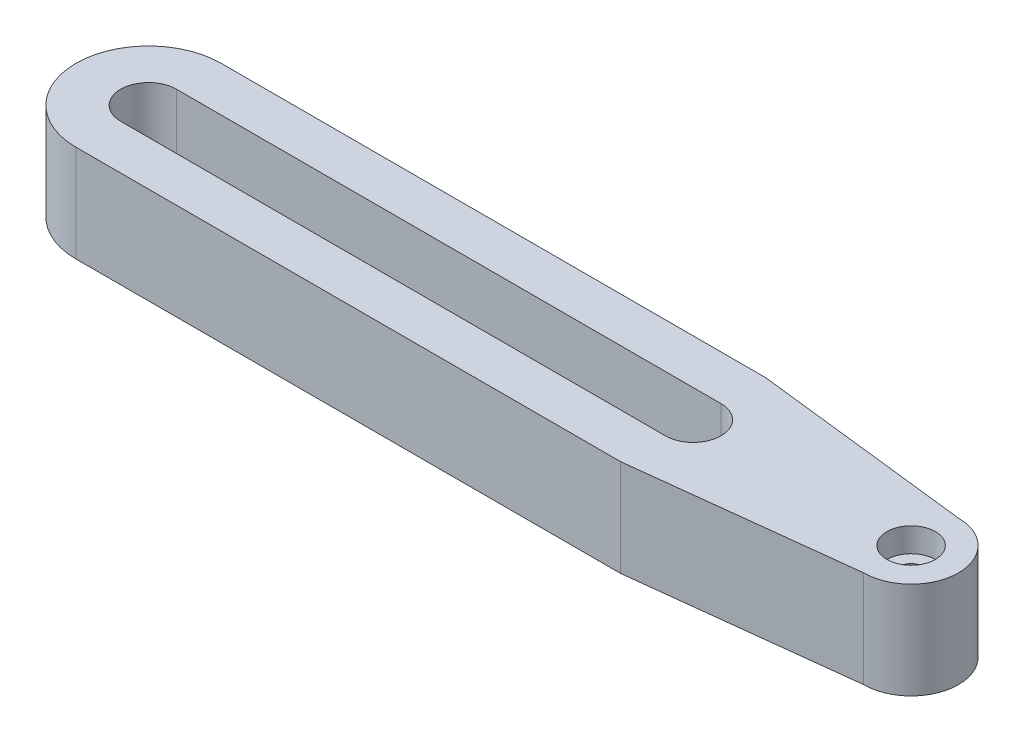
SolidWorks part; units mm, degrees
ref_plane "Front Plane" through (0, 0, 0) normal (0, 0, 1) x (1, 0, 0)
ref_plane "Top Plane" through (0, 0, 0) normal (0, 1, 0) x (1, 0, 0)
ref_plane "Right Plane" through (0, 0, 0) normal (1, 0, 0) x (0, 0, -1)
sketch "Sketch1" plane through (0, 0, 0) normal (0, 1, 0) x (1, 0, 0)
  line L0 (0, 0) -> (45, 0) construction
  line L1 (0, 6) -> (45, 6)
  line L2 (0, -6) -> (45, -6)
  line L3 (45, -6) -> (63, -3.9143)
  line L4 (45, 6) -> (63, 3.9143)
  line L5 (0, 0) -> (45, 0) construction
  line L6 (0, 2.3) -> (45, 2.3)
  line L7 (0, -2.3) -> (45, -2.3)
  arc A0 (0, 6) -> (0, -6) centre (0, 0) ccw
  arc A3 (63, -3.9143) -> (63, 3.9143) centre (63, 0) ccw
  arc A4 (0, 2.3) -> (0, -2.3) centre (0, 0) ccw
  arc A5 (45, -2.3) -> (45, 2.3) centre (45, 0) ccw
  point P3 (22.5, 0)
  point P15 (22.5, 0)
  dimension "D5" = 63
  dimension "D1" = 45
  dimension "D3" = 12
  dimension "D4" = 4.6
  dimension "D6" = 45
  dimension "D7" = 6.609
  dimension "D8" = 6.609
extrude "Boss-Extrude1" add sketch "Sketch1" along normal blind 8
sketch "Sketch2" plane through (0, 8, 0) normal (0, 1, 0) x (1, 0, 0)
  circle A0 centre (63, 0) radius 2
  dimension "D1" = 4
extrude "Cut-Extrude1" cut sketch "Sketch2" against normal blind 2
sketch "Sketch3" plane through (0, 0, 0) normal (0, -1, 0) x (1, 0, 0)
  circle A0 centre (63, 0) radius 1
  dimension "D1" = 2
extrude "Cut-Extrude2" cut sketch "Sketch3" against normal through all
equation "\"1\"= \"代号代号\""
equation "\"2\"= \"名称代号\""
